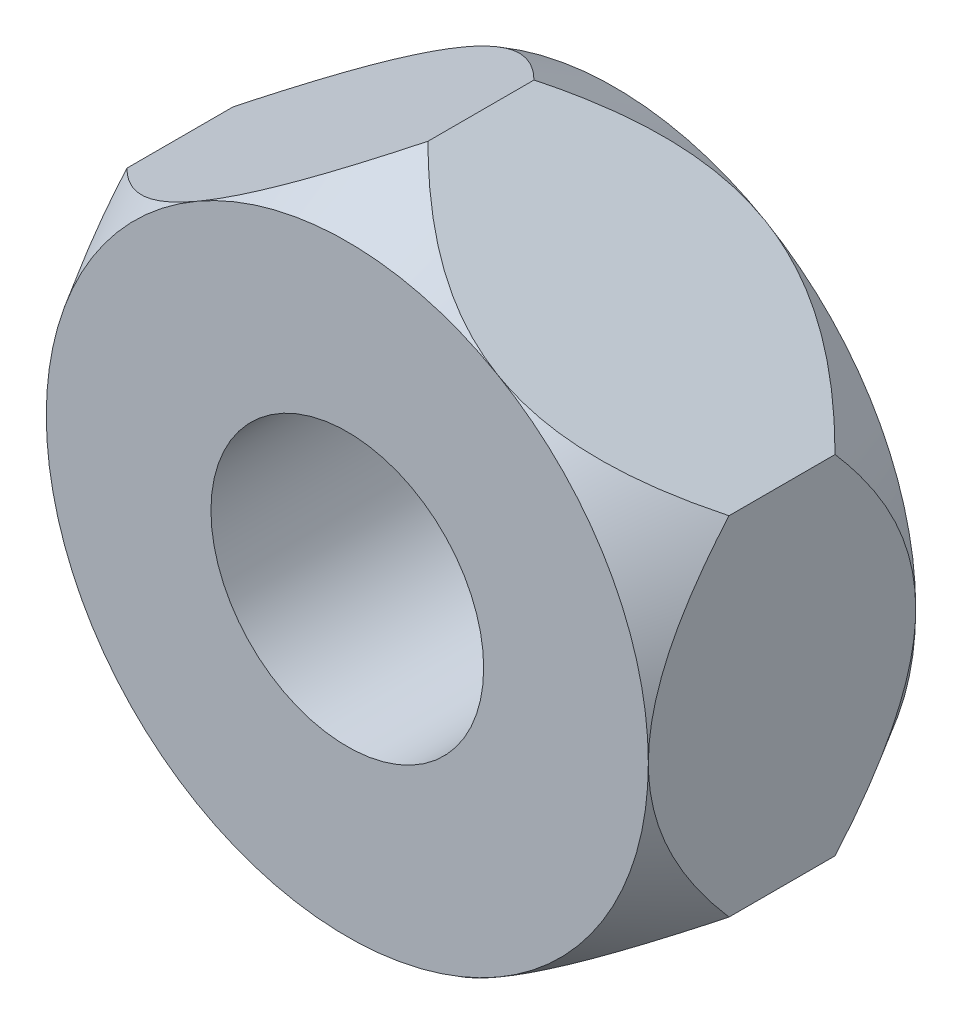
from build123d import *

# Parameters (mm, degrees)
BOSS_EXTRUDE1_DEPTH     = 5
SKETCH2_OUTSIDE_W       = 43.226
SKETCH2_OUTSIDE_H       = 46.71
SKETCH2_OUTSIDE_R       = 11.258330249
CUT_EXTRUDE1_DEPTH      = 10
CUT_EXTRUDE1_DRAFT      = -30
MIRROR1_COPY_1_SKETCH_W = 43.226
MIRROR1_COPY_1_SKETCH_H = 46.71
MIRROR1_COPY_1_SKETCH_R = 11.258330249
MIRROR1_COPY_1_DEPTH    = 10
MIRROR1_COPY_1_DRAFT    = -30
M12_TAPPED_HOLE3_D      = 10.2
M12_TAPPED_HOLE3_DEPTH  = 38.75


with BuildPart() as part:
    # Sketch1 → Boss-Extrude1 (new, symmetric)
    with BuildSketch(Plane.XY):
        Polygon((0, 13), (-11.258330249, 6.5), (-11.258330249, -6.5), (0, -13), (11.258330249, -6.5), (11.258330249, 6.5), align=None)
    extrude(amount=BOSS_EXTRUDE1_DEPTH, both=True)


with BuildPart() as cut_extrude1_tool:
    # Sketch2 outside → Cut-Extrude1 (with draft: the straight prism first)
    with BuildSketch(Plane.XY.offset(5)):
        Rectangle(SKETCH2_OUTSIDE_W, SKETCH2_OUTSIDE_H)
        Circle(SKETCH2_OUTSIDE_R, mode=Mode.SUBTRACT)
    extrude(amount=-CUT_EXTRUDE1_DEPTH)
    # Cut-Extrude1: the draft: its side faces are tilted about the plane it starts from
    cut_extrude1_sides = [cut_extrude1_tool.faces().sort_by_distance(p)[0] for p in [
        (0, -23.355, 0),
        (21.613, 0, 0),
        (0, 23.355, 0),
        (-21.613, 0, 0),
        (-11.258330249, 0, 0),
    ]]
    draft(cut_extrude1_sides, Plane.XY.offset(5), CUT_EXTRUDE1_DRAFT)


with BuildPart() as part_1:
    add(part.part)

    # Cut-Extrude1: cut by cut_extrude1_tool
    add(cut_extrude1_tool.part, mode=Mode.SUBTRACT)


with BuildPart() as mirror1_copy_1_tool:
    # Mirror1 copy 1 sketch → Mirror1 copy 1 (with draft: the straight prism first)
    with BuildSketch(Plane(origin=(0, 0, -5), x_dir=(1, 0, 0), z_dir=(0, 0, -1))):
        Rectangle(MIRROR1_COPY_1_SKETCH_W, MIRROR1_COPY_1_SKETCH_H)
        Circle(MIRROR1_COPY_1_SKETCH_R, mode=Mode.SUBTRACT)
    extrude(amount=-MIRROR1_COPY_1_DEPTH)
    # Mirror1 copy 1: the draft: its side faces are tilted about the plane it starts from
    mirror1_copy_1_sides = [mirror1_copy_1_tool.faces().sort_by_distance(p)[0] for p in [
        (0, -23.355, 0),
        (21.613, 0, 0),
        (0, 23.355, 0),
        (-21.613, 0, 0),
        (-11.258330249, 0, 0),
    ]]
    draft(mirror1_copy_1_sides, Plane(origin=(0, 0, -5), x_dir=(1, 0, 0), z_dir=(0, 0, -1)), MIRROR1_COPY_1_DRAFT)


with BuildPart() as part_2:
    add(part_1.part)

    # Mirror1 copy 1: cut by mirror1_copy_1_tool
    add(mirror1_copy_1_tool.part, mode=Mode.SUBTRACT)

    # M12 Tapped Hole3
    with Locations(Plane.XY.offset(5)):
        with Locations((0, 0)):
            Hole(M12_TAPPED_HOLE3_D / 2, depth=M12_TAPPED_HOLE3_DEPTH)


solid = part_2.part
